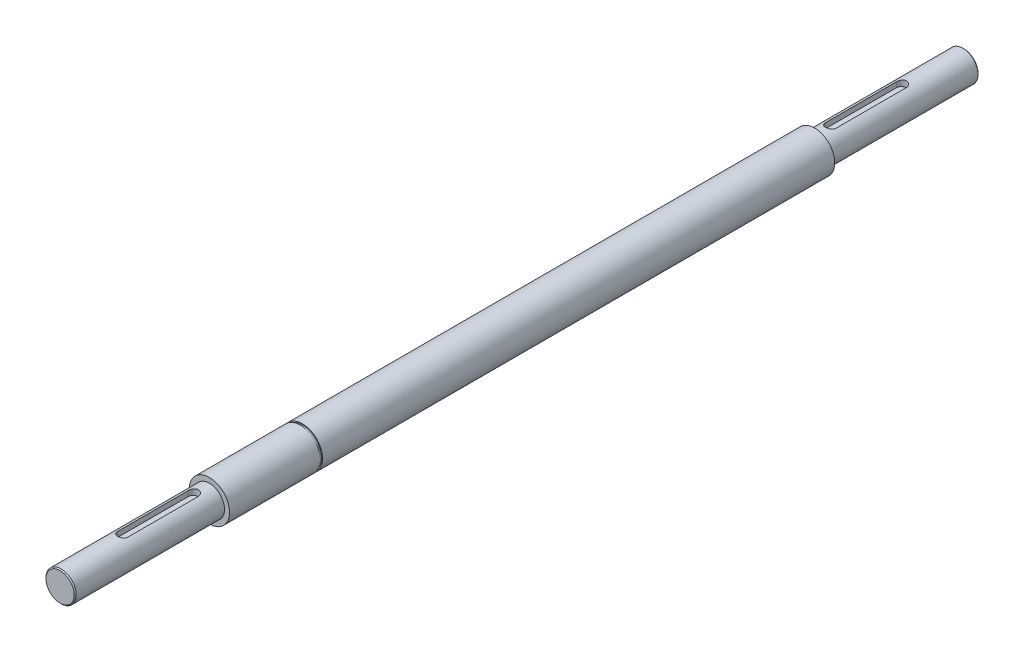
from build123d import *

# Parameters (mm, degrees)
SKETCH_1_R          = 10
EXTRUDE_1_DEPTH     = 300
SKETCH_2_R          = 6
EXTRUDE_2_DEPTH     = 74
EXTRUDE_START       = 74
SKETCH_3_R          = 6
EXTRUDE_3_DEPTH     = 74
SKETCH_4_R          = 7.5
EXTRUDE_4_DEPTH     = 74
SKETCH_5_R          = 7.5
EXTRUDE_5_DEPTH     = 74
CUT_EXTRUDE_1_DEPTH = 3
CHAMFER_1_SIZE      = 0.5
SKETCH_8_R          = 12.5
SKETCH_8_R_2        = 9.5
CUT_EXTRUDE_2_DEPTH = 1.1


with BuildPart() as part:
    # 草图1 → 凸台-拉伸1 (new body)
    with BuildSketch(Plane.XY):
        with Locations(Location((0, 0, 0), (0, 0, 90))):
            Circle(SKETCH_1_R)
    extrude(amount=EXTRUDE_1_DEPTH)

    # 草图2 → 凸台-拉伸2 (add)
    with BuildSketch(Plane(origin=(0, 0, 0), x_dir=(-1, 0, 0), z_dir=(0, 0, -1))):
        Circle(SKETCH_2_R)
    extrude(amount=EXTRUDE_2_DEPTH)

    # 草图3 → 凸台-拉伸3 (add)
    with BuildSketch(Plane.XY.offset(300).offset(EXTRUDE_START)):
        Circle(SKETCH_3_R)
    extrude(amount=-EXTRUDE_3_DEPTH)

    # 草图4 → 凸台-拉伸4 (add)
    with BuildSketch(Plane.XY.offset(300)):
        Circle(SKETCH_4_R)
    extrude(amount=EXTRUDE_4_DEPTH)

    # 草图5 → 凸台-拉伸5 (add)
    with BuildSketch(Plane(origin=(0, 0, 0), x_dir=(-1, 0, 0), z_dir=(0, 0, -1)).offset(EXTRUDE_START)):
        with Locations(Location((0, 0, 0), (0, 0, 180))):
            Circle(SKETCH_5_R)
    extrude(amount=-EXTRUDE_5_DEPTH)

    # 草图7 → 切除-拉伸1 (cut)
    with BuildSketch(Plane(origin=(0, 7.5, 0), x_dir=(1, 0, 0), z_dir=(0, 1, 0))):
        with BuildLine():
            Line((-2.5, 8), (-2.5, 43))
            ThreePointArc((-2.5, 43), (0, 45.5), (2.5, 43))
            Line((2.5, 43), (2.5, 8))
            ThreePointArc((2.5, 8), (0, 5.5), (-2.5, 8))
        make_face()
        with BuildLine():
            Line((2.5, -308), (2.5, -343))
            ThreePointArc((2.5, -343), (0, -345.5), (-2.5, -343))
            Line((-2.5, -343), (-2.5, -308))
            ThreePointArc((-2.5, -308), (0, -305.5), (2.5, -308))
        make_face()
    extrude(amount=-CUT_EXTRUDE_1_DEPTH, mode=Mode.SUBTRACT)

    # 倒角1
    chamfer_1_edges = [part.edges().sort_by_distance(p)[0] for p in [
        (-7.5, 0, 374),
        (-7.5, 0, -74),
    ]]
    chamfer(chamfer_1_edges, length=CHAMFER_1_SIZE)

    # 草图8 → 切除-拉伸2 (cut)
    with BuildSketch(Plane(origin=(0, 0, 255), x_dir=(-1, 0, 0), z_dir=(0, 0, -1))):
        Circle(SKETCH_8_R)
        with Locations(Location((0, 0, 0), (0, 0, 90))):
            Circle(SKETCH_8_R_2, mode=Mode.SUBTRACT)
    extrude(amount=CUT_EXTRUDE_2_DEPTH, mode=Mode.SUBTRACT)


solid = part.part
